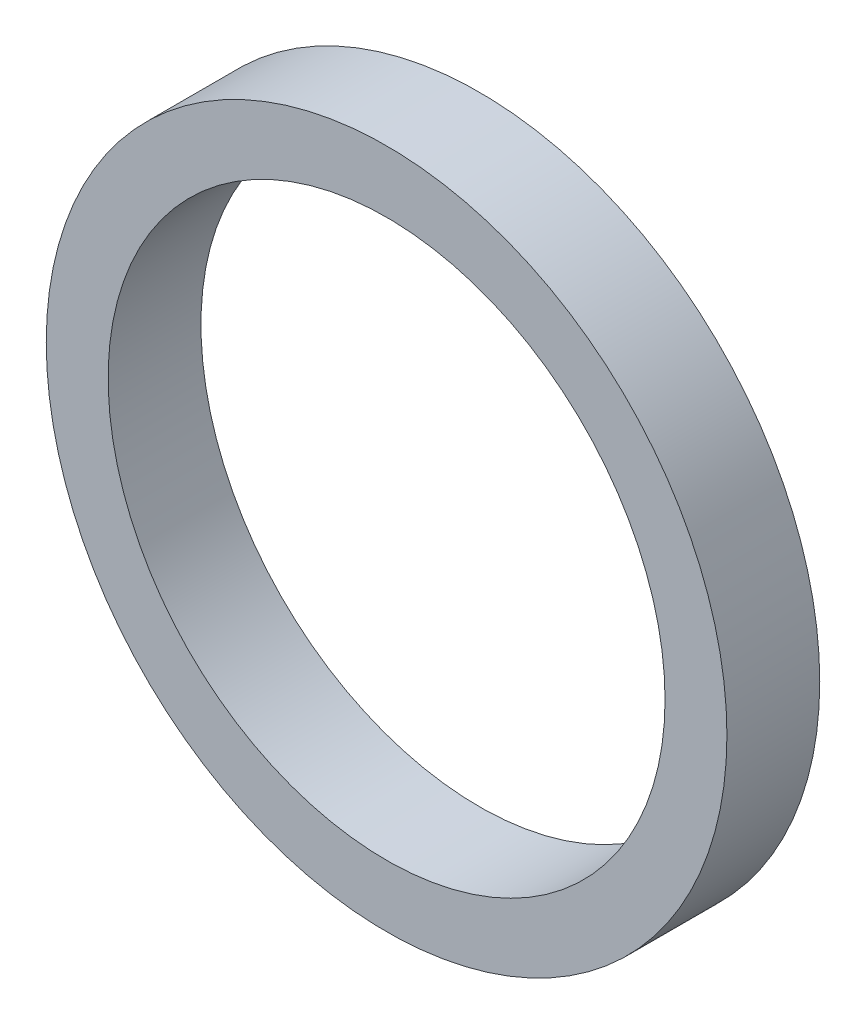
SolidWorks part; units mm, degrees
material "橡胶"
ref_plane "前视基准面" through (0, 0, 0) normal (0, 0, 1) x (1, 0, 0)
ref_plane "上视基准面" through (0, 0, 0) normal (0, 1, 0) x (1, 0, 0)
ref_plane "右视基准面" through (0, 0, 0) normal (1, 0, 0) x (0, 0, -1)
sketch "草图1" plane through (0, 0, 0) normal (0, 0, 1) x (1, 0, 0)
  circle A0 centre (0, 0) radius 90
  circle A1 centre (0, 0) radius 110
extrude "凸台-拉伸2" add sketch "草图1" along normal blind 30
